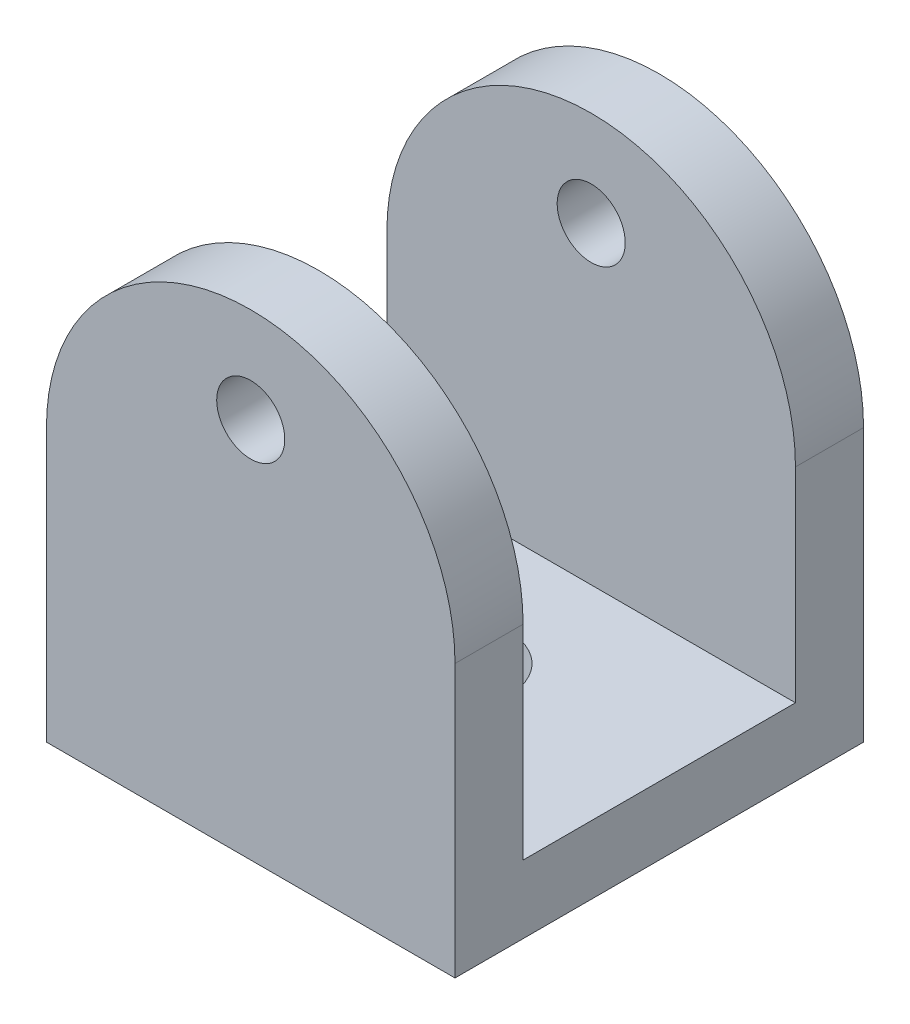
SolidWorks part; units mm, degrees
ref_plane "前视" through (0, 0, 0) normal (0, 0, 1) x (1, 0, 0)
ref_plane "上视" through (0, 0, 0) normal (0, 1, 0) x (1, 0, 0)
ref_plane "右视" through (0, 0, 0) normal (1, 0, 0) x (0, 0, -1)
sketch "草图1" plane through (0, 0, 0) normal (0, 0, 1) x (1, 0, 0)
  line L1 (0, 0) -> (30, 0)
  line L2 (0, 0) -> (0, 40)
  line L3 (0, 40) -> (30, 40)
  line L4 (30, 0) -> (30, 40)
  dimension "D1" = 30
  dimension "D2" = 40
extrude "凸台-拉伸1" add sketch "草图1" along normal blind 30
sketch "草图4" plane through (30, 0, 0) normal (1, 0, 0) x (0, 0, -1)
  line L0 (-30, 40) -> (0, 40) construction
  line L1 (0, 0) -> (0, 40) construction
  line L2 (-25, 40) -> (-5, 40)
  line L3 (-25, 40) -> (-25, 5)
  line L4 (-25, 5) -> (-5, 5)
  line L5 (-5, 40) -> (-5, 5)
  dimension "D1" = 20
  dimension "D2" = 5
  dimension "D3" = 35
extrude "切除-拉伸1" cut sketch "草图4" against normal blind 40
sketch "草图5" plane through (0, 0, 0) normal (0, 0, -1) x (-1, 0, 0)
  line L0 (-30, 20) -> (-30, 40)
  line L1 (-30, 0) -> (-30, 40) construction
  line L2 (-30, 40) -> (0, 40)
  line L3 (0, 40) -> (0, 20)
  line L4 (0, 40) -> (0, 0) construction
  arc A0 (0, 20) -> (-30, 20) centre (-15, 20) ccw
extrude "切除-拉伸2" cut sketch "草图5" against normal blind 40
sketch "草图6" plane through (0, 0, 0) normal (0, 0, -1) x (-1, 0, 0)
  line L0 (0, 0) -> (-30, 0) construction
  line L1 (-30, 0) -> (-30, 20) construction
  circle A0 centre (-15, 28) radius 2.5
  dimension "D1" = 28
  dimension "D2" = 15
extrude "切除-拉伸3" cut sketch "草图6" against normal blind 40
sketch "草图7" plane through (0, 0, 0) normal (0, -1, 0) x (1, 0, 0)
  line L0 (30, 15) -> (-4.9646, 15) construction
  line L1 (30, 30) -> (30, 0) construction
  line L2 (15, 30) -> (15, -11.8938) construction
  line L3 (0, 30) -> (30, 30) construction
  circle A0 centre (15, 15) radius 4
extrude "切除-拉伸4" cut sketch "草图7" against normal blind 40
